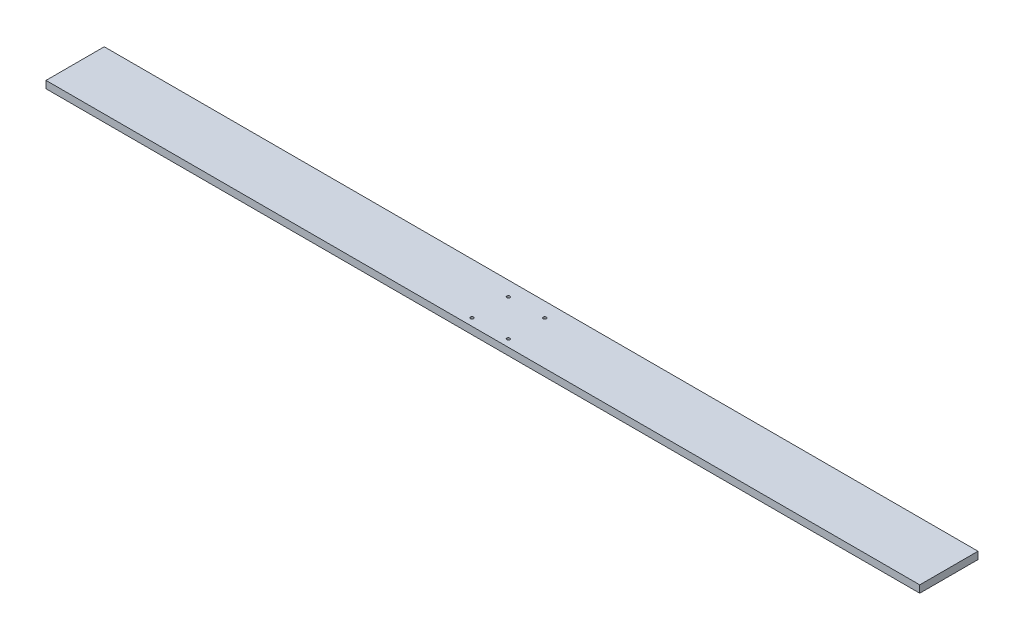
SolidWorks part; units mm, degrees
ref_plane "前视基准面" through (0, 0, 0) normal (0, 0, 1) x (1, 0, 0)
ref_plane "上视基准面" through (0, 0, 0) normal (0, 1, 0) x (1, 0, 0)
ref_plane "右视基准面" through (0, 0, 0) normal (1, 0, 0) x (0, 0, -1)
other "Configuration Table"
sketch "草图2" plane through (0, 0, 0) normal (0, 1, 0) x (1, 0, 0)
  line L1 (-600, 40) -> (600, 40)
  line L2 (-600, 40) -> (-600, -40)
  line L3 (-600, -40) -> (600, -40)
  line L4 (600, 40) -> (600, -40)
  line L5 (-600, 40) -> (600, -40) construction
  line L6 (-600, -40) -> (600, 40) construction
  point P0 (0, 0)
  dimension "D1" = 1200
  dimension "D2" = 80
extrude "凸台-拉伸1" add sketch "草图2" along normal mid plane 10
sketch "草图4" plane through (0, 5, 0) normal (0, 1, 0) x (1, 0, 0)
  line L0 (-600, -40) -> (600, -40) construction
  line L1 (-25, 20) -> (25, 20) construction
  line L2 (-25, 20) -> (-25, -30) construction
  line L3 (-25, -30) -> (25, -30) construction
  line L4 (25, 20) -> (25, -30) construction
  line L5 (-25, 20) -> (25, -30) construction
  line L6 (-25, -30) -> (25, 20) construction
  circle A0 centre (-25, 20) radius 2.1
  circle A1 centre (25, 20) radius 2.1
  circle A2 centre (25, -30) radius 2.1
  circle A3 centre (-25, -30) radius 2.1
  point P0 (0, -5)
  dimension "D4" = 4.2
  dimension "D1" = 50
  dimension "D2" = 50
  dimension "D3" = 10
extrude "切除-拉伸1" cut sketch "草图4" against normal blind 26
